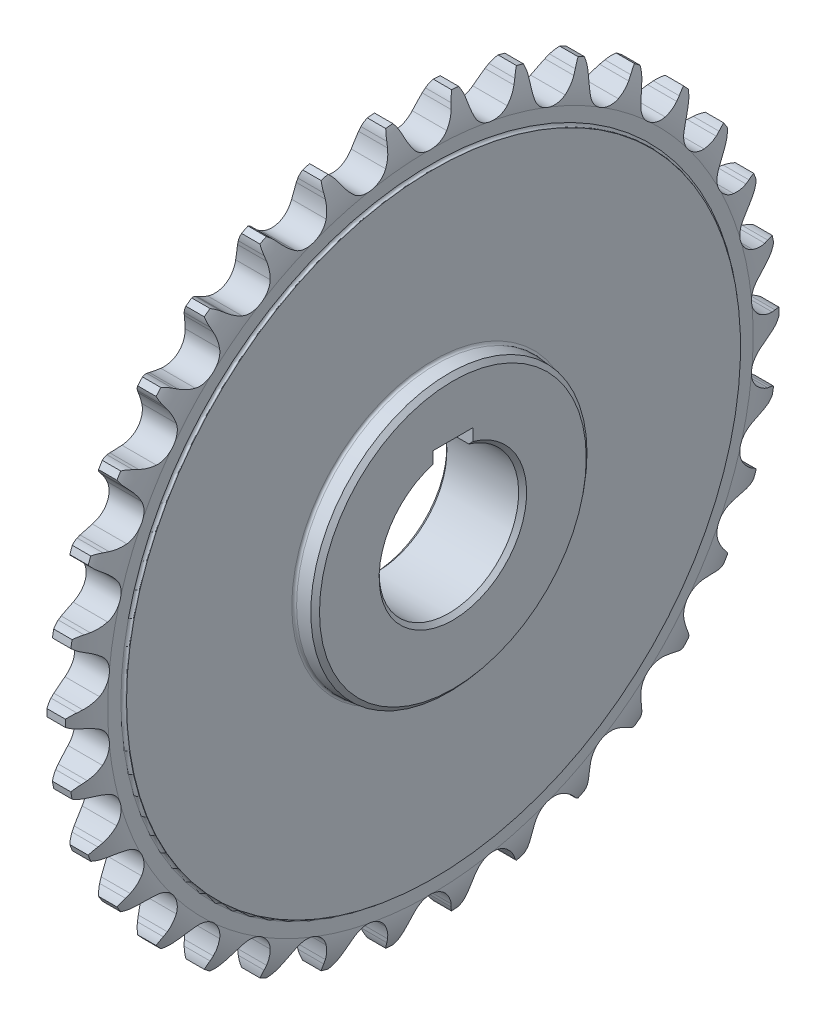
SolidWorks part; units mm, degrees
ref_plane "前视基准面" through (0, 0, 0) normal (0, 0, 1) x (1, 0, 0)
ref_plane "上视基准面" through (0, 0, 0) normal (0, 1, 0) x (1, 0, 0)
ref_plane "右视基准面" through (0, 0, 0) normal (1, 0, 0) x (0, 0, -1)
sketch "草图1" plane through (0, 0, 0) normal (0, 0, 1) x (1, 0, 0)
  line L0 (-7.9375, 0) -> (7.9375, 0) construction
  line L1 (-5.15, 17.5) -> (-5.15, 77)
  line L2 (-5.15, 77) -> (-5.006, 77)
  line L3 (-4.371, 77.635) -> (-4.371, 80.9462)
  line L4 (-2.3072, 89.5) -> (2.3072, 89.5)
  line L5 (4.371, 80.9462) -> (4.371, 77.635)
  line L6 (5.006, 77) -> (5.15, 77)
  line L7 (5.15, 77) -> (5.15, 17.5)
  line L8 (5.15, 17.5) -> (-5.15, 17.5)
  line L9 (0, 0) -> (0, 89.5) construction
  line L10 (-3.7701, 86.0262) -> (3.7701, 86.0262) construction
  line L11 (-3.7701, -86.0262) -> (3.7701, -86.0262) construction
  line L12 (7.9375, 0) -> (41.9375, 0) construction
  line L13 (-4.371, 80.9462) -> (3.7984, 80.9462) construction
  line L14 (-4.371, -80.9462) -> (3.7984, -80.9462) construction
  line L15 (41.9375, 0) -> (52.0975, 0) construction
  line L16 (52.0975, 0) -> (67.1875, 0) construction
  line L17 (67.1875, 0) -> (76.5875, 0) construction
  line L18 (76.5875, 0) -> (94.6975, 0) construction
  arc A0 (-2.3072, 89.5) -> (-4.371, 80.9462) centre (11.4886, 81.6457) ccw
  arc A1 (2.3072, 89.5) -> (4.371, 80.9462) centre (-11.4886, 81.6457) cw
  arc A2 (4.371, 77.635) -> (5.006, 77) centre (5.006, 77.635) ccw
  arc A3 (-5.006, 77) -> (-4.371, 77.635) centre (-5.006, 77.635) ccw
  point P30 (4.371, 77)
  point P33 (-4.371, 77)
  dimension "rx" = 15.875
  dimension "D3" = 0.635
  dimension "d" = 172.0525
  dimension "p" = 15.875
  dimension "z" = 34
  dimension "da" = 179
  dimension "df" = 161.8925
  dimension "dr" = 10.16
  dimension "dk" = 35
  dimension "dg" = 154
  dimension "h" = 15.09
  dimension "bf1" = 8.742
  dimension "b1" = 9.4
  dimension "ba" = 2.0638
  dimension "pt" = 18.11
  dimension "t" = 10.3
revolve "旋转1" add sketch "草图1" angle 360 about L0
sketch "草图2" plane through (0, 0, 0) normal (1, 0, 0) x (0, 0, -1)
  line L0 (0, 0) -> (0, 89.5) construction
  line L1 (0, 0) -> (-8.258, 89.1182) construction
  line L2 (0, 0) -> (-16.4456, 87.9761) construction
  line L3 (4.13, 82.9406) -> (23.5451, 68.4349) construction
  line L4 (5.938, 86.2583) -> (-6.5113, 90.8911) construction
  line L5 (0, 0) -> (8.258, 89.1182) construction
  line L6 (5.938, 86.2583) -> (6.3412, 87.3419)
  line L7 (-5.938, 86.2583) -> (-6.3412, 87.3419)
  circle A0 centre (0, 0) radius 89.5 construction
  arc A1 (4.13, 82.9406) -> (-4.13, 82.9406) centre (0, 86.0262) cw
  arc A2 (4.13, 82.9406) -> (5.938, 86.2583) centre (-6.5113, 90.8911) ccw
  arc A3 (7.3604, 89.1968) -> (6.3412, 87.3419) centre (13.1517, 84.8076) ccw
  arc A4 (-4.13, 82.9406) -> (-5.938, 86.2583) centre (6.5113, 90.8911) cw
  arc A5 (-7.3604, 89.1968) -> (-6.3412, 87.3419) centre (-13.1517, 84.8076) cw
  arc A7 (7.3604, 89.1968) -> (-7.3604, 89.1968) centre (0, 0) ccw
  dimension "r1" = 5.1554
  dimension "r3" = 7.2667
  dimension "D1" = 10.588
  dimension "D2" = 5.294
  dimension "α/2" = 53.235
  dimension "M" = 6.5113
  dimension "T" = 4.8649
  dimension "β" = 16.353
  dimension "γ/2" = 15.118
  dimension "bc" = 1.1562
extrude "切除-拉伸1" cut sketch "草图2" against normal mid plane 10.3
pattern_circular "阵列(圆周)1" count 34 over 360 about axis through (0, 0, 0) along (1, 0, 0) of "切除-拉伸1"
sketch "草图4" plane through (-5.15, 0, 0) normal (-1, 0, 0) x (0, 0, 1)
  line L1 (-5, 16.7705) -> (5, 16.7705)
  line L2 (-5, 16.7705) -> (-5, 20.8)
  line L3 (-5, 20.8) -> (5, 20.8)
  line L4 (5, 16.7705) -> (5, 20.8)
  circle A0 centre (0, 0) radius 17.5 construction
  point P6 (1.7, 20.8)
  dimension "D1" = 20.8
  dimension "键槽宽度" = 10
  dimension "t1" = 3.3
sketch "草图5" plane through (0, 0, 0) normal (0, 0, 1) x (1, 0, 0)
  line L1 (-10, 17.5) -> (10, 17.5)
  line L2 (-10, 17.5) -> (-10, 34.5539)
  line L3 (-10, 34.5539) -> (-5.15, 34.9782)
  line L4 (10, 17.5) -> (10, 34.5539)
  line L6 (0, 0) -> (0, -4.2677) construction
  line L7 (0, 0) -> (-10.4728, 0) construction
  line L8 (-5.15, 17.5) -> (-5.15, 77) construction
  line L9 (-5.15, 34.9782) -> (5.15, 34.9782)
  line L10 (5.15, 77) -> (5.15, 17.5) construction
  line L11 (5.15, 34.9782) -> (10, 34.5539)
  dimension "D1" = 5
  dimension "L" = 20
  dimension "H" = 17.0539
revolve "旋转2" add sketch "草图5" angle 360 about L7
extrude "切除-拉伸2" cut sketch "草图4" against normal through all
mirror "镜向1" about plane through (0, 0, 0) normal (1, 0, 0) of "切除-拉伸2"
fillet "圆角1" radius 0.635 2 edges at (5.15, 0, -34.9782) (-5.15, 0, -34.9782)
chamfer "倒角1" distance 1 angle 45 4 edges at (10, -17.5, 0) (10, 0, -34.5539) (-10, -17.5, 0) (-10, 0, -34.5539)
